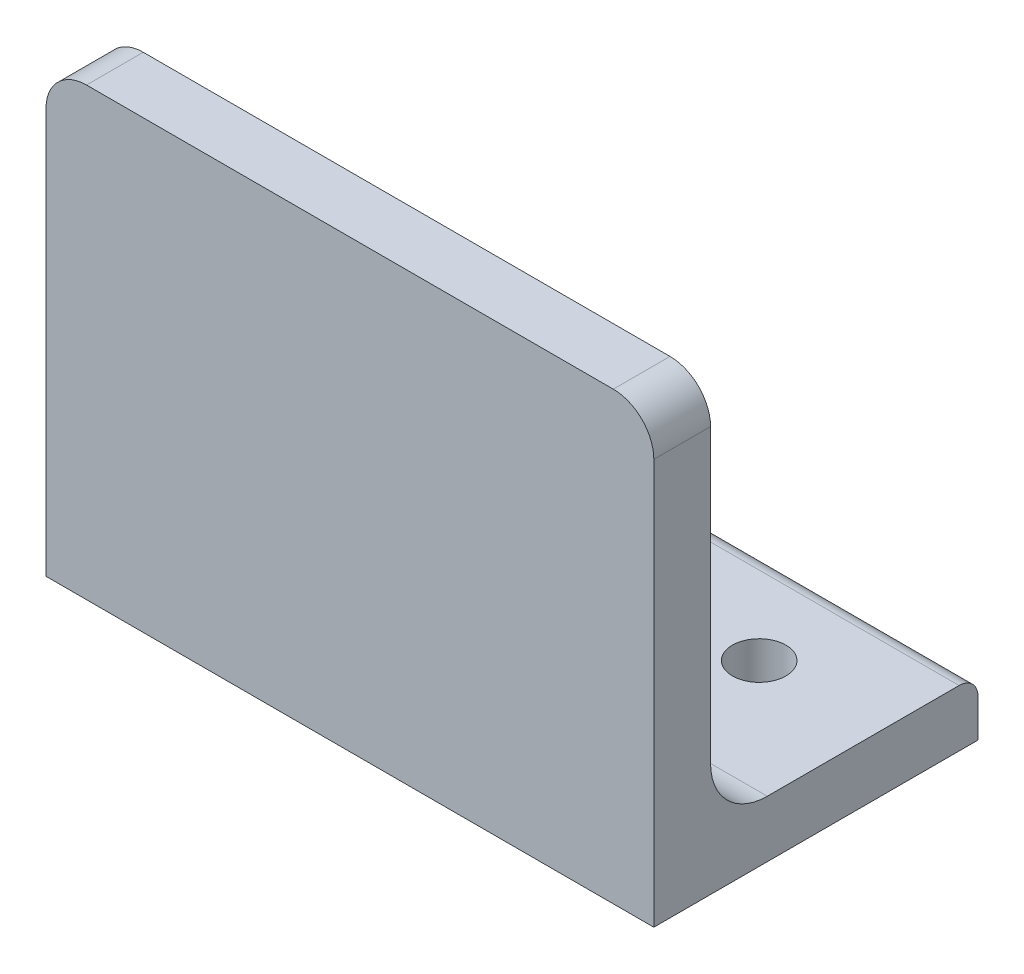
from build123d import *

# Parameters (mm, degrees)
UNEQUAL_ANGLE_STEEL_6_3_4_1_DEPTH = 75
M6_CLEARANCE_HOLE1_D              = 6.6
M6_CLEARANCE_HOLE1_DEPTH          = 20
M6_CLEARANCE_HOLE1_TIP            = 1.982840043
CUT_EXTRUDE1_DEPTH                = 106.80170131
CUT_EXTRUDE1_DEPTH_BACK           = 106.80170131
SKETCH8_W                         = 14
SKETCH8_H                         = 16
FILLET1_R                         = 5


with BuildPart() as part:
    # Sketch11 → Unequal Angle Steel 6.3-4(1) (new body)
    with BuildSketch(Plane.YZ):
        with BuildLine():
            Line((63, 0), (0, 0))
            Line((0, 0), (0, -40))
            Line((0, -40), (4.666666667, -40))
            ThreePointArc((4.666666667, -40), (6.316582489, -39.316582489), (7, -37.666666667))
            Line((7, -37.666666667), (7, -14))
            ThreePointArc((7, -14), (9.050252532, -9.050252532), (14, -7))
            Line((14, -7), (60.666666667, -7))
            ThreePointArc((60.666666667, -7), (62.316582489, -6.316582489), (63, -4.666666667))
            Line((63, -4.666666667), (63, 0))
        make_face()
    extrude(amount=UNEQUAL_ANGLE_STEEL_6_3_4_1_DEPTH)

    # M6 Clearance Hole1
    with Locations(Plane.XZ):
        with Locations((15, -28), (60, -28)):
            Hole(M6_CLEARANCE_HOLE1_D / 2, depth=M6_CLEARANCE_HOLE1_DEPTH)
            with Locations((0, 0, -(M6_CLEARANCE_HOLE1_DEPTH + M6_CLEARANCE_HOLE1_TIP / 2))):  # 118° drill point
                Cone(0, M6_CLEARANCE_HOLE1_D / 2, M6_CLEARANCE_HOLE1_TIP, mode=Mode.SUBTRACT)

    # Sketch8 → Cut-Extrude1 (cut, two sides: drawn at the far end of the back side and taken through both)
    with BuildSketch(Plane(origin=(75, 0, 0), x_dir=(0, 0, -1), z_dir=(1, 0, 0)).offset(-CUT_EXTRUDE1_DEPTH_BACK)):
        with Locations((0, 63)):
            Rectangle(SKETCH8_W, SKETCH8_H)
    extrude(amount=CUT_EXTRUDE1_DEPTH + CUT_EXTRUDE1_DEPTH_BACK, mode=Mode.SUBTRACT)

    # Fillet1
    fillet1_edges = [part.edges().sort_by_distance(p)[0] for p in [
        (0, 55, -3.5),
        (75, 55, -3.5),
    ]]
    fillet(fillet1_edges, radius=FILLET1_R)


solid = part.part
